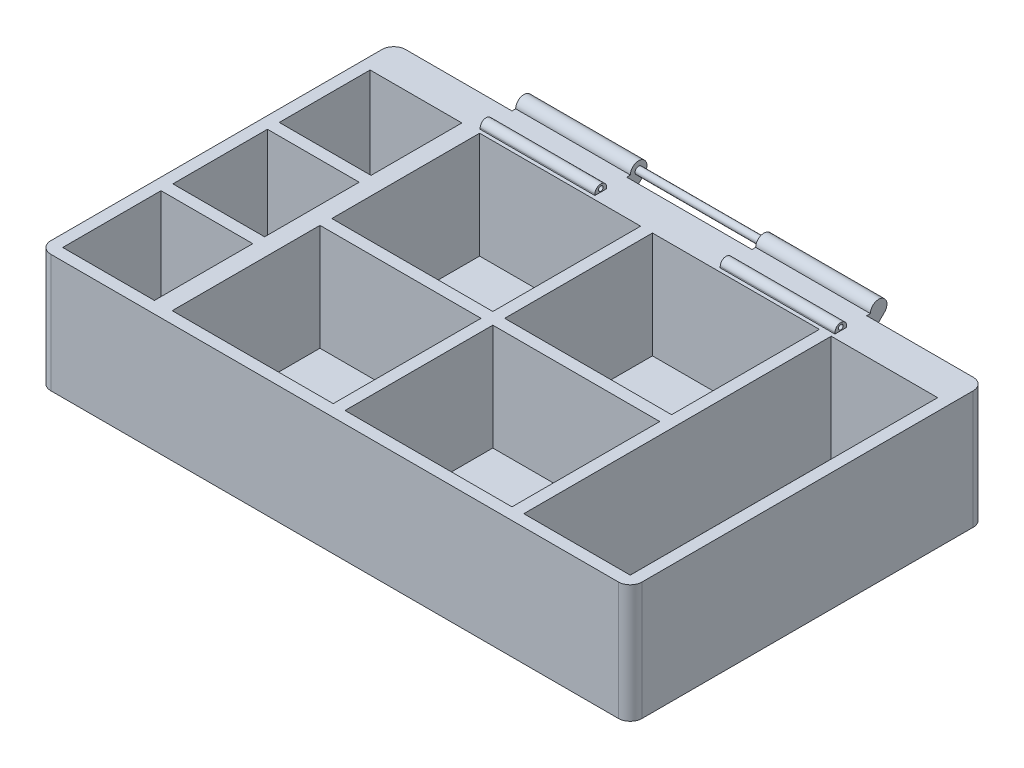
from build123d import *
from build123d.topology import SkipClean

# Parameters (mm, degrees)
SKETCH1_W                 = 50
SKETCH1_H                 = 30
BOSS_EXTRUDE2_DEPTH       = 10
SHELL3_T                  = -1
SHELL3_THICKNESS_2_FACE_W = 48
SHELL3_THICKNESS_2_FACE_H = 9
SHELL3_THICKNESS_2_DEPTH  = 2
BOSS_EXTRUDE3_DEPTH       = 10
SKETCH3_R                 = 3.1
BOSS_EXTRUDE12_DEPTH      = 1.5
CUT_EXTRUDE2_DEPTH        = 1.5
CIRPATTERN4_COUNT         = 6
SKETCH22_R                = 3.1
BOSS_EXTRUDE13_DEPTH      = 1.5
CUT_EXTRUDE3_DEPTH        = 1.5
CIRPATTERN5_COUNT         = 6
SKETCH27_R                = 3.1
BOSS_EXTRUDE14_DEPTH      = 1.5
CUT_EXTRUDE4_DEPTH        = 1.5
CIRPATTERN6_COUNT         = 6
SKETCH30_W                = 1
SKETCH30_H                = 12.5
SKETCH30_H_2              = 26
BOSS_EXTRUDE15_DEPTH      = 9
SKETCH31_W                = 0.5
SKETCH31_H                = 26
BOSS_EXTRUDE16_DEPTH      = 10
SKETCH32_R                = 0.3
BOSS_EXTRUDE19_DEPTH      = 15
BOSS_EXTRUDE20_START      = 15
SKETCH35_R                = 0.3
BOSS_EXTRUDE20_DEPTH      = 15
SKETCH37_W                = 10.6
SKETCH37_H                = 3.741104567
CUT_EXTRUDE5_DEPTH        = 2.5
SKETCH40_R                = 0.3
BOSS_EXTRUDE21_DEPTH      = 15
FILLET1_R                 = 1
SKETCH66_W                = 30
SKETCH66_H                = 1
BOSS_EXTRUDE22_DEPTH      = 0.1
BOSS_EXTRUDE23_DEPTH      = 30
SKETCH68_R                = 0.2
CUT_EXTRUDE8_DEPTH        = 34.5
SKETCH69_W                = 10.6
SKETCH69_H                = 3.310548063
CUT_EXTRUDE9_DEPTH        = 34.5


with BuildPart() as part:
    # Sketch1 → Boss-Extrude2 (new body)
    with BuildSketch(Plane(origin=(0, 0, 0), x_dir=(1, 0, 0), z_dir=(0, 1, 0))):
        Rectangle(SKETCH1_W, SKETCH1_H)
    extrude(amount=BOSS_EXTRUDE2_DEPTH)

    # Shell3
    shell3_openings = [part.faces().sort_by_distance(p)[0] for p in [
        (0, 10, 0),
    ]]
    offset(amount=SHELL3_T, openings=shell3_openings, kind=Kind.INTERSECTION)

    # Shell3 thickness 2 face (on inner face of the shell) → Shell3 thickness 2 (add)
    with BuildSketch(Plane(origin=(0, 5.5, -14), x_dir=(-1, 0, 0), z_dir=(0, 0, -1))):
        Rectangle(SHELL3_THICKNESS_2_FACE_W, SHELL3_THICKNESS_2_FACE_H)
    extrude(amount=-SHELL3_THICKNESS_2_DEPTH)

    # Sketch2 → Boss-Extrude3 (add)
    with BuildSketch(Plane(origin=(0, 0, 0), x_dir=(1, 0, 0), z_dir=(0, 1, 0))):
        Polygon((-15.24058795, 12.317112), (-16.24058795, 12.317112), (-16.24058795, 4.317112), (-24.24058795, 4.317112), (-24.24058795, 3.317112), (-16.24058795, 3.317112), (-16.24058795, -4.682888), (-24.24058795, -4.682888), (-24.24058795, -5.682888), (-16.24058795, -5.682888), (-16.24058795, -14.110921237), (-15.24058795, -14.110921237), align=None)
    extrude(amount=BOSS_EXTRUDE3_DEPTH)

    # Sketch3 → Boss-Extrude12 (add)
    with BuildSketch(Plane(origin=(0, 1, 0), x_dir=(1, 0, 0), z_dir=(0, 1, 0))):
        with Locations(Location((-20.120293975, 8.158556, 0), (0, 0, 270))):
            Circle(SKETCH3_R)
    extrude(amount=BOSS_EXTRUDE12_DEPTH)

    # Sketch18 → Cut-Extrude2 (cut)
    with BuildSketch(Plane(origin=(0, 2.5, 0), x_dir=(1, 0, 0), z_dir=(0, 1, 0))):
        with BuildLine():
            Line((-18.343158931, 10.572969651), (-18.292649957, 10.641591085))
            ThreePointArc((-18.292649957, 10.641591085), (-19.016172181, 11.037212102), (-19.818678555, 11.226906375))
            Line((-19.818678555, 11.226906375), (-19.862912417, 11.145420071))
            ThreePointArc((-19.862912417, 11.145420071), (-19.063535099, 10.964061823), (-18.343158931, 10.572969651))
        make_face()
    cut_extrude2 = extrude(amount=-CUT_EXTRUDE2_DEPTH, mode=Mode.SUBTRACT)

    # CirPattern4: Cut-Extrude2 ×6 about axis
    cirpattern4_axis = Axis((-20.120293975, 0, -8.158556), (0, 1, 0))
    for i in range(1, CIRPATTERN4_COUNT):
        add(cut_extrude2.rotate(cirpattern4_axis, i * 360 / CIRPATTERN4_COUNT), mode=Mode.SUBTRACT)

    # Sketch22 → Boss-Extrude13 (add)
    with BuildSketch(Plane(origin=(0, 1, 0), x_dir=(1, 0, 0), z_dir=(0, 1, 0))):
        with Locations(Location((-20.120293975, -0.682888, 0), (0, 0, 270))):
            Circle(SKETCH22_R)
    extrude(amount=BOSS_EXTRUDE13_DEPTH)

    # Sketch23 → Cut-Extrude3 (cut)
    with BuildSketch(Plane(origin=(0, 2.5, 0), x_dir=(1, 0, 0), z_dir=(0, 1, 0))):
        with BuildLine():
            Line((-19.481811993, 2.248381479), (-19.436483295, 2.456485436))
            ThreePointArc((-19.436483295, 2.456485436), (-18.499115293, 2.093421016), (-17.725070876, 1.452071043))
            Line((-17.725070876, 1.452071043), (-17.88079423, 1.313268531))
            ThreePointArc((-17.88079423, 1.313268531), (-18.607249441, 1.907613156), (-19.481811993, 2.248381479))
        make_face()
    cut_extrude3 = extrude(amount=-CUT_EXTRUDE3_DEPTH, mode=Mode.SUBTRACT)

    # CirPattern5: Cut-Extrude3 ×6 about axis
    cirpattern5_axis = Axis((-20.120293975, 0, 0.682888), (0, 1, 0))
    for i in range(1, CIRPATTERN5_COUNT):
        add(cut_extrude3.rotate(cirpattern5_axis, i * 360 / CIRPATTERN5_COUNT), mode=Mode.SUBTRACT)

    # Sketch27 → Boss-Extrude14 (add)
    with BuildSketch(Plane(origin=(0, 1, 0), x_dir=(1, 0, 0), z_dir=(0, 1, 0))):
        with Locations(Location((-20.120293975, -9.841444, 0), (0, 0, 270))):
            Circle(SKETCH27_R)
    extrude(amount=BOSS_EXTRUDE14_DEPTH)

    # Sketch28 → Cut-Extrude4 (cut)
    with BuildSketch(Plane(origin=(0, 2.5, 0), x_dir=(1, 0, 0), z_dir=(0, 1, 0))):
        with BuildLine():
            Line((-22.757767397, -11.271036231), (-23.112348525, -11.463230178))
            ThreePointArc((-23.112348525, -11.463230178), (-22.435626904, -12.288964796), (-21.509349026, -12.819812333))
            Line((-21.509349026, -12.819812333), (-21.413761565, -12.548276391))
            ThreePointArc((-21.413761565, -12.548276391), (-22.186911965, -12.016091117), (-22.757767397, -11.271036231))
        make_face()
    cut_extrude4 = extrude(amount=-CUT_EXTRUDE4_DEPTH, mode=Mode.SUBTRACT)

    # CirPattern6: Cut-Extrude4 ×6 about axis
    cirpattern6_axis = Axis((-20.120293975, 0, 9.841444), (0, 1, 0))
    for i in range(1, CIRPATTERN6_COUNT):
        add(cut_extrude4.rotate(cirpattern6_axis, i * 360 / CIRPATTERN6_COUNT), mode=Mode.SUBTRACT)

    # Sketch30 → Boss-Extrude15 (add)
    with BuildSketch(Plane(origin=(0, 1, 0), x_dir=(1, 0, 0), z_dir=(0, 1, 0))):
        Polygon((-1.121602155, -1.5), (-1.121602155, -0.5), (-15.24058795, -0.5), (-15.24058795, -1), (-15.24058795, -1.5), align=None)
        Polygon((13.997383641, -1), (13.997383641, -0.5), (-0.121602155, -0.5), (-0.121602155, -1.5), (13.997383641, -1.5), align=None)
        Polygon((-0.621602155, -0.5), (-0.121602155, -0.5), (-0.121602155, 12), (-1.121602155, 12), (-1.121602155, -0.5), align=None)
        with Locations((-0.621602155, -7.75)):
            Rectangle(SKETCH30_W, SKETCH30_H)
        with Locations((14.497383641, -1)):
            Rectangle(SKETCH30_W, SKETCH30_H_2)
        Polygon((-0.121602155, -1.5), (-0.121602155, -0.5), (-0.621602155, -0.5), (-1.121602155, -0.5), (-1.121602155, -1.5), align=None)
    extrude(amount=BOSS_EXTRUDE15_DEPTH)

    # Sketch31 → Boss-Extrude16 (add)
    with BuildSketch(Plane(origin=(0, 10, 0), x_dir=(1, 0, 0), z_dir=(0, 1, 0))):
        with Locations((-14.99058795, -1)):
            Rectangle(SKETCH31_W, SKETCH31_H)
    extrude(amount=-BOSS_EXTRUDE16_DEPTH)

    # Sketch32 → Boss-Extrude19 (add)
    with BuildSketch(Plane(origin=(0, 0, 0), x_dir=(0, 0, -1), z_dir=(1, 0, 0))):
        with BuildLine():
            Line((15.310548063, 10), (15, 10))
            Line((15, 10), (15, 7.99944207))
            Line((15, 7.99944207), (16.502372161, 9.501894533))
            ThreePointArc((16.502372161, 9.501894533), (16.280476879, 10.645862551), (15.310548063, 10))
        make_face()
        with Locations((16.010548063, 10)):
            Circle(SKETCH32_R, mode=Mode.SUBTRACT)
    extrude(amount=BOSS_EXTRUDE19_DEPTH)

    # Sketch35 → Boss-Extrude20 (add)
    # profile 1 of 2: a face of its own
    with SkipClean():  # the faces are left unmerged after this step: merging them gives an invalid solid
        with BuildSketch(Plane.ZY.offset(BOSS_EXTRUDE20_START)):
            with BuildLine():
                ThreePointArc((-15.310548063, 10), (-15.740619247, 9.354137449), (-16.502372161, 9.501894533))
                Line((-16.502372161, 9.501894533), (-15, 7.99944207))
                Line((-15, 7.99944207), (-15, 10))
                Line((-15, 10), (-15.310548063, 10))
            make_face()
        # profile 2 of 2: a face of its own
        with BuildSketch(Plane.ZY.offset(BOSS_EXTRUDE20_START)):
            with BuildLine():
                ThreePointArc((-15.310548063, 10), (-16.280476879, 10.645862551), (-16.502372161, 9.501894533))
                ThreePointArc((-16.502372161, 9.501894533), (-15.740619247, 9.354137449), (-15.310548063, 10))
            make_face()
            with Locations((-16.010548063, 10)):
                Circle(SKETCH35_R, mode=Mode.SUBTRACT)
        extrude(amount=-BOSS_EXTRUDE20_DEPTH)

    # Sketch37 → Cut-Extrude5 (cut, symmetric)
    with BuildSketch(Plane(origin=(0, 10, 0), x_dir=(1, 0, 0), z_dir=(0, 1, 0))):
        with Locations((0, 16.870552284)):
            Rectangle(SKETCH37_W, SKETCH37_H)
    extrude(amount=CUT_EXTRUDE5_DEPTH, both=True, mode=Mode.SUBTRACT)

    # Sketch40 → Boss-Extrude21 (add, symmetric)
    with BuildSketch(Plane(origin=(0, 0, 0), x_dir=(0, 0, -1), z_dir=(1, 0, 0))):
        with Locations(Location((16.010548063, 10, 0), (0, 0, 180))):
            Circle(SKETCH40_R)
    extrude(amount=BOSS_EXTRUDE21_DEPTH, both=True)

    # Fillet1
    fillet1_edges = [part.edges().sort_by_distance(p)[0] for p in [
        (25, 5, 15),
        (-25, 5, 15),
        (-25, 5, -15),
        (25, 5, -15),
    ]]
    fillet(fillet1_edges, radius=FILLET1_R)

    # Sketch66 → Boss-Extrude22 (add)
    with BuildSketch(Plane(origin=(0, 10, 0), x_dir=(1, 0, 0), z_dir=(0, 1, 0))):
        with Locations((0, 12.810548063)):
            Rectangle(SKETCH66_W, SKETCH66_H)
    extrude(amount=BOSS_EXTRUDE22_DEPTH)

    # Sketch67 → Boss-Extrude23 (add)
    with BuildSketch(Plane.ZY.offset(15)):
        with BuildLine():
            Line((-13.310548063, 10.1), (-12.310548063, 10.1))
            ThreePointArc((-12.310548063, 10.1), (-12.810548063, 10.6), (-13.310548063, 10.1))
        make_face()
    extrude(amount=-BOSS_EXTRUDE23_DEPTH)

    # Sketch68 → Cut-Extrude8 (cut)
    with BuildSketch(Plane.ZY.offset(15)):
        with Locations((-12.810548063, 10.255419354)):
            Circle(SKETCH68_R)
    extrude(amount=-CUT_EXTRUDE8_DEPTH, mode=Mode.SUBTRACT)

    # Sketch69 → Cut-Extrude9 (cut)
    with BuildSketch(Plane(origin=(0, 10, 0), x_dir=(1, 0, 0), z_dir=(0, 1, 0))):
        with Locations((0, 13.655274031)):
            Rectangle(SKETCH69_W, SKETCH69_H)
    extrude(amount=CUT_EXTRUDE9_DEPTH, mode=Mode.SUBTRACT)


solid = part.part
